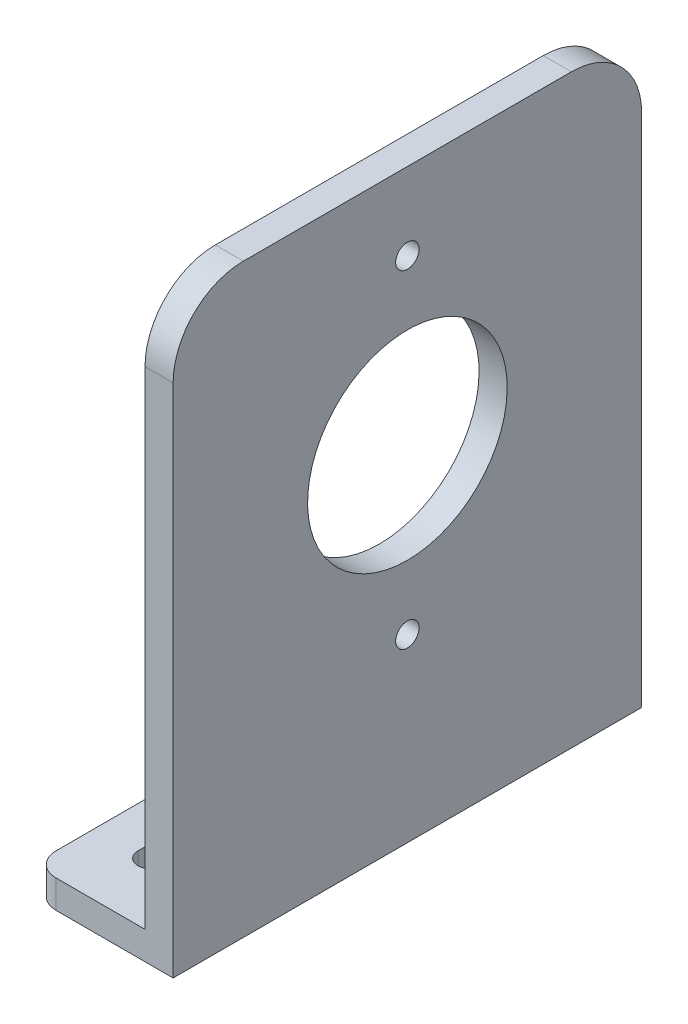
from build123d import *

# Parameters (mm, degrees)
BOSS_EXTRUDE_1_DEPTH = 100
CUT_EXTRUDE_1_DEPTH  = 266.035846632
SKETCH_3_R           = 42.6
SKETCH_3_R_2         = 5
CUT_EXTRUDE_2_DEPTH  = 274.50319925
FILLET_1_R           = 30
FILLET_2_R           = 10


with BuildPart() as part:
    # Sketch 1 → Boss-Extrude 1 (new, symmetric)
    with BuildSketch(Plane.XY):
        Polygon((-60, 0), (0, 0), (0, 250), (-12, 250), (-12, 12), (-60, 12), align=None)
    extrude(amount=BOSS_EXTRUDE_1_DEPTH, both=True)

    # Sketch 2 → Cut-Extrude 1 (cut, through all)
    with BuildSketch(Plane(origin=(0, 12, 0), x_dir=(1, 0, 0), z_dir=(0, 1, 0))):
        with BuildLine():
            Line((-42.5, 67.5), (-42.5, 72.5))
            ThreePointArc((-42.5, 72.5), (-37, 78), (-31.5, 72.5))
            Line((-31.5, 72.5), (-31.5, 67.5))
            ThreePointArc((-31.5, 67.5), (-37, 62), (-42.5, 67.5))
        make_face()
        with BuildLine():
            Line((-42.5, -67.5), (-42.5, -72.5))
            ThreePointArc((-42.5, -72.5), (-37, -78), (-31.5, -72.5))
            Line((-31.5, -72.5), (-31.5, -67.5))
            ThreePointArc((-31.5, -67.5), (-37, -62), (-42.5, -67.5))
        make_face()
    extrude(amount=-CUT_EXTRUDE_1_DEPTH, mode=Mode.SUBTRACT)

    # Sketch 3 → Cut-Extrude 2 (cut, through all)
    with BuildSketch(Plane.ZY.offset(12)):
        with Locations(Location((0, 147, 0), (0, 0, 270))):
            Circle(SKETCH_3_R)
        with Locations(Location((0, 217, 0), (0, 0, 270))):
            Circle(SKETCH_3_R_2)
        with Locations(Location((0, 77, 0), (0, 0, 90))):
            Circle(SKETCH_3_R_2)
    extrude(amount=-CUT_EXTRUDE_2_DEPTH, mode=Mode.SUBTRACT)

    # Fillet 1
    fillet_1_edges = [part.edges().sort_by_distance(p)[0] for p in [
        (-6, 250, 100),
        (-6, 250, -100),
    ]]
    fillet(fillet_1_edges, radius=FILLET_1_R)

    # Fillet 2
    fillet_2_edges = [part.edges().sort_by_distance(p)[0] for p in [
        (-60, 6, 100),
        (-60, 6, -100),
    ]]
    fillet(fillet_2_edges, radius=FILLET_2_R)


solid = part.part
